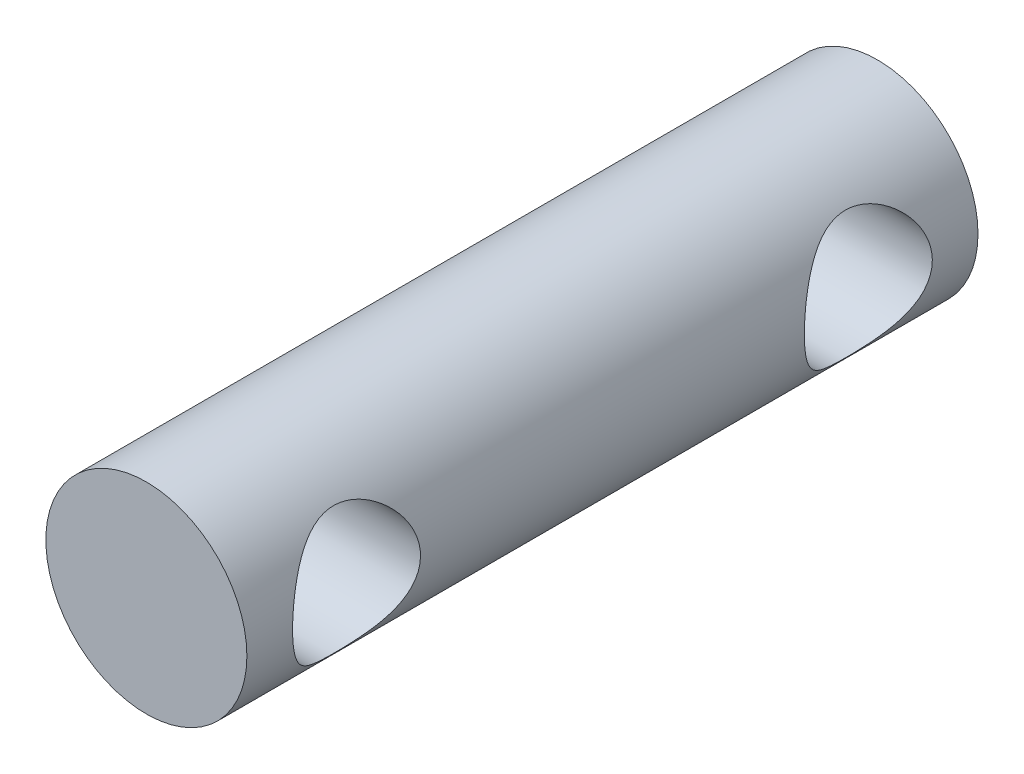
SolidWorks part; units mm, degrees
ref_plane "前视基准面" through (0, 0, 0) normal (0, 0, 1) x (1, 0, 0)
ref_plane "上视基准面" through (0, 0, 0) normal (0, 1, 0) x (1, 0, 0)
ref_plane "右视基准面" through (0, 0, 0) normal (1, 0, 0) x (0, 0, -1)
sketch "草图1" plane through (0, 0, 0) normal (0, 0, 1) x (1, 0, 0)
  circle A0 centre (0, 0) radius 5.5
  dimension "D1" = 11
extrude "凸台-拉伸1" add sketch "草图1" along normal mid plane 40
sketch "草图2" plane through (0, 0, 0) normal (1, 0, 0) x (0, 0, -1)
  line L0 (0, 4.3788) -> (0, -7.8652) construction
  circle A0 centre (-14, 0) radius 3.5
  circle A1 centre (14, 0) radius 3.5
  dimension "D1" = 28
  dimension "D2" = 7
extrude "切除-拉伸1" cut sketch "草图2" against normal mid plane 40
